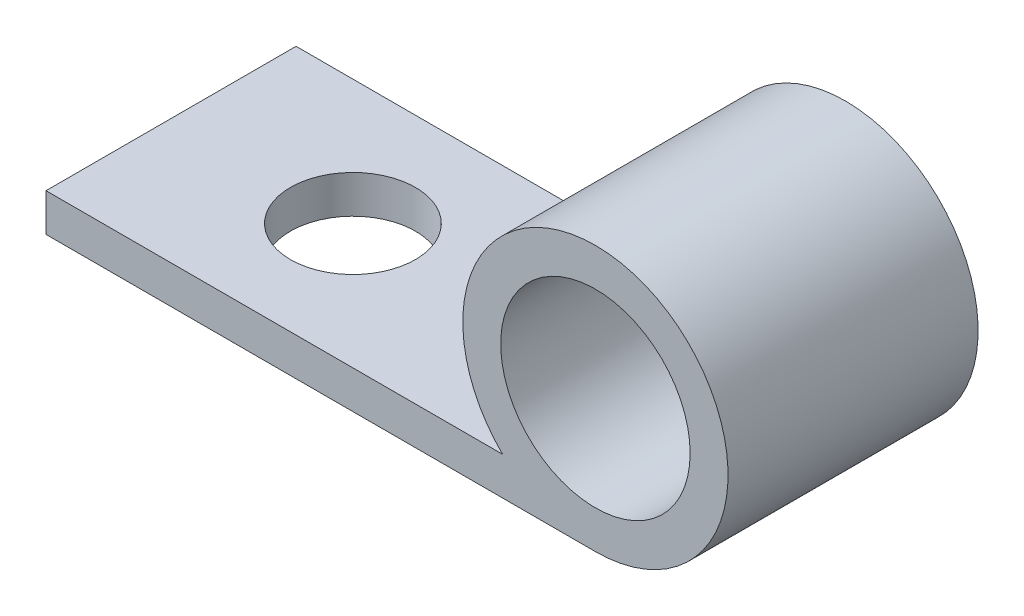
from build123d import *

# Parameters (mm, degrees)
SKETCH_1_R          = 2.5
EXTRUDE_1_DEPTH     = 3.3
SKETCH_2_R          = 1.65
CUT_EXTRUDE_1_DEPTH = 6.6


with BuildPart() as part:
    # 草图1 → 凸台-拉伸1 (new, symmetric)
    with BuildSketch(Plane.XY):
        with BuildLine():
            Line((0, 1), (0, 0))
            Line((0, 0), (14.5, 0))
            ThreePointArc((14.5, 0), (15.822875656, 6.740370349), (12.050510257, 1))
            Line((12.050510257, 1), (0, 1))
        make_face()
        with Locations((14.5, 3.5)):
            Circle(SKETCH_1_R, mode=Mode.SUBTRACT)
    extrude(amount=EXTRUDE_1_DEPTH, both=True)

    # 草图2 → 切除-拉伸1 (cut)
    with BuildSketch(Plane(origin=(0, 1, 0), x_dir=(1, 0, 0), z_dir=(0, 1, 0))):
        with Locations(Location((4.8, 0, 0), (0, 0, 270))):
            Circle(SKETCH_2_R)
    extrude(amount=-CUT_EXTRUDE_1_DEPTH, mode=Mode.SUBTRACT)


solid = part.part
